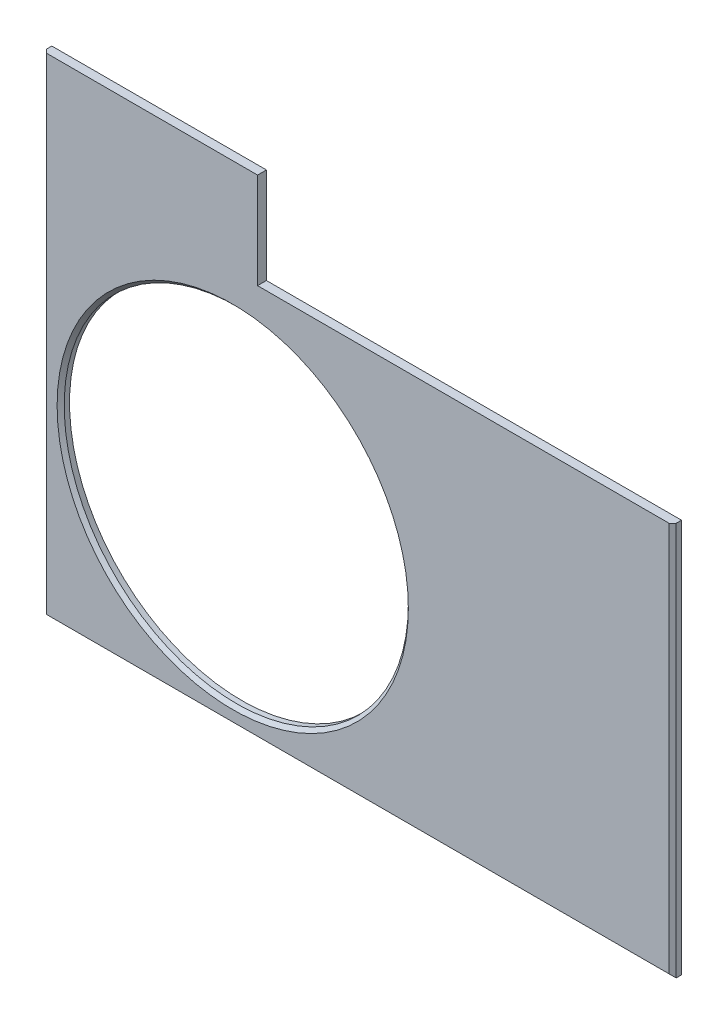
SolidWorks part; units mm, degrees
material "Q235"
ref_plane "Front Plane" through (0, 0, 0) normal (0, 0, 1) x (1, 0, 0)
ref_plane "Top Plane" through (0, 0, 0) normal (0, 1, 0) x (1, 0, 0)
ref_plane "Right Plane" through (0, 0, 0) normal (1, 0, 0) x (0, 0, -1)
sketch "Sketch1" plane through (0, 0, 0) normal (0, 0, 1) x (1, 0, 0)
  line L0 (0, 0) -> (1775, 0)
  line L1 (1775, 0) -> (1775, 1110)
  line L2 (1775, 1110) -> (605, 1110)
  line L3 (605, 1110) -> (605, 1380)
  line L4 (605, 1380) -> (0, 1380)
  line L5 (0, 1380) -> (0, 0)
  circle A1 centre (535, 535) radius 485
  dimension "D5" = 535
  dimension "D6" = 970
  dimension "D7" = 535
  dimension "D1" = 1380
  dimension "D2" = 1775
  dimension "D3" = 605
  dimension "D4" = 1110
extrude "Boss-Extrude1" add sketch "Sketch1" along normal blind 25
chamfer "Chamfer1" distance 10 angle 45 4 edges at (1775, 555, 25) (887.5, 0, 25) (0, 690, 25) (1020, 535, 25)
